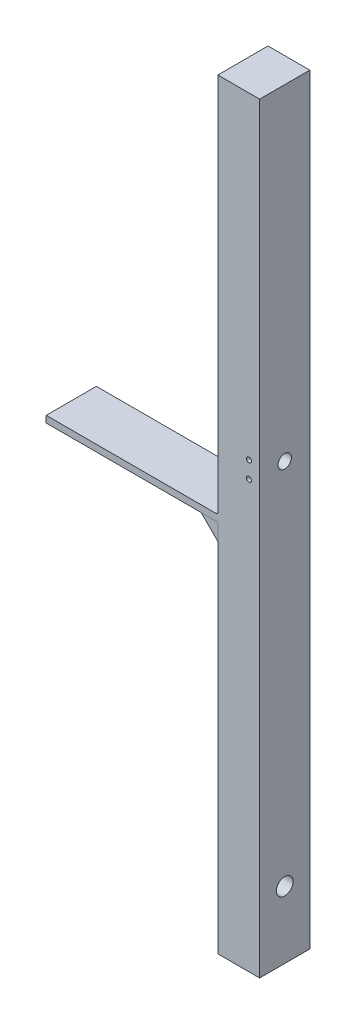
from build123d import *

# Parameters (mm, degrees)
EXTRUDE_2_DEPTH     = 15
SKETCH_2_R          = 5
SKETCH_2_R_2        = 4
CUT_EXTRUDE_1_DEPTH = 66
SKETCH_3_W          = 102.6
SKETCH_3_H          = 4
EXTRUDE_3_DEPTH     = 30
SKETCH_4_W          = 25
SKETCH_4_H          = 30
EXTRUDE_4_DEPTH     = 155
SKETCH_5_R          = 1
CUT_EXTRUDE_2_DEPTH = 10
SKETCH_6_R          = 1.5
CUT_EXTRUDE_3_DEPTH = 10
GUSSET_1_THICKNESS  = 5
GUSSET_2_THICKNESS  = 5
FILLET_1_R          = 1


with BuildPart() as part:
    # 草图1 → 凸台-拉伸2 (new, symmetric)
    with BuildSketch(Plane.XY):
        Polygon((0, 0), (0, 246.032566337), (25, 246.032566337), (25, -38.967433663), (25, -53.967433663), (0, -53.967433663), align=None)
    extrude(amount=EXTRUDE_2_DEPTH, both=True)

    # 草图2 → 切除-拉伸1 (cut, symmetric)
    with BuildSketch(Plane.ZY):
        with Locations(Location((0, -13.967433663, 0), (0, 0, 270))):
            Circle(SKETCH_2_R)
        with Locations(Location((0, 206.032566337, 0), (0, 0, 270))):
            Circle(SKETCH_2_R_2)
    extrude(amount=CUT_EXTRUDE_1_DEPTH, both=True, mode=Mode.SUBTRACT)

    # 草图3 → 凸台-拉伸3 (add)
    with BuildSketch(Plane(origin=(0, 0, -15), x_dir=(-1, 0, 0), z_dir=(0, 0, -1))):
        with Locations((51.3, 171.532566337)):
            Rectangle(SKETCH_3_W, SKETCH_3_H)
    extrude(amount=-EXTRUDE_3_DEPTH)

    # 草图4 → 凸台-拉伸4 (add)
    with BuildSketch(Plane(origin=(0, 246.032566337, 0), x_dir=(1, 0, 0), z_dir=(0, 1, 0))):
        with Locations((12.5, 0)):
            Rectangle(SKETCH_4_W, SKETCH_4_H)
    extrude(amount=EXTRUDE_4_DEPTH)

    # 草图5 → 切除-拉伸2 (cut)
    with BuildSketch(Plane(origin=(0, 0, -15), x_dir=(-1, 0, 0), z_dir=(0, 0, -1))):
        with Locations((-18.6, 201.032566337)):
            Circle(SKETCH_5_R)
        with Locations((-18.6, 211.032566337)):
            Circle(SKETCH_5_R)
    extrude(amount=-CUT_EXTRUDE_2_DEPTH, mode=Mode.SUBTRACT)

    # 草图6 → 切除-拉伸3 (cut)
    with BuildSketch(Plane.XY.offset(15)):
        with Locations((18.6, 201.032566337)):
            Circle(SKETCH_6_R)
        with Locations((18.6, 211.032566337)):
            Circle(SKETCH_6_R)
    extrude(amount=-CUT_EXTRUDE_3_DEPTH, mode=Mode.SUBTRACT)

    # 圆角1
    fillet_1_edges = [part.edges().sort_by_distance(p)[0] for p in [
        (0, 173.532566337, 0),
    ]]
    fillet(fillet_1_edges, radius=FILLET_1_R)


with BuildPart() as body_2:
    # Gusset 1: a gusset: a plate 5.0 thick in the corner of two members, its outline drawn in place
    gusset_1_outline = Wire([Line((0, 169.532566337, -10), (-10, 169.532566337, -10)), Line((-10, 169.532566337, -10), (0, 159.532566337, -10)), Line((0, 159.532566337, -10), (0, 169.532566337, -10))])
    add(extrude(Face(gusset_1_outline), amount=GUSSET_1_THICKNESS, dir=(0, 0, -1)))


with BuildPart() as body_3:
    # Gusset 2: a gusset: a plate 5.0 thick in the corner of two members, its outline drawn in place
    gusset_2_outline = Wire([Line((0, 169.532566337, 15), (-10, 169.532566337, 15)), Line((-10, 169.532566337, 15), (0, 159.532566337, 15)), Line((0, 159.532566337, 15), (0, 169.532566337, 15))])
    add(extrude(Face(gusset_2_outline), amount=GUSSET_2_THICKNESS, dir=(0, 0, -1)))


solid = Compound([part.part, body_2.part, body_3.part])
